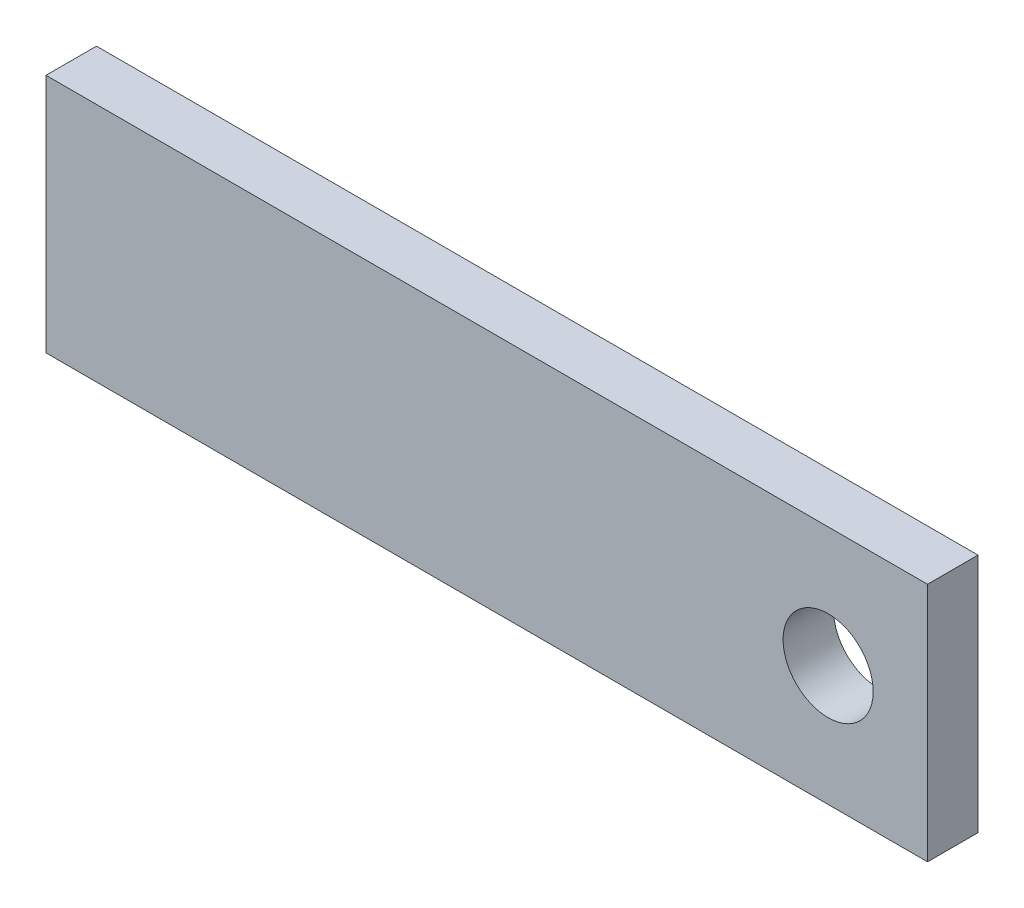
SolidWorks part; units mm, degrees
material "普通碳钢"
ref_plane "Front Plane" through (0, 0, 0) normal (0, 0, 1) x (1, 0, 0)
ref_plane "Top Plane" through (0, 0, 0) normal (0, 1, 0) x (1, 0, 0)
ref_plane "Right Plane" through (0, 0, 0) normal (1, 0, 0) x (0, 0, -1)
sketch "Sketch1" plane through (0, 0, 0) normal (0, 0, 1) x (1, 0, 0)
  line L1 (-123.952, 19.05) -> (15.748, 19.05)
  line L2 (-123.952, 19.05) -> (-123.952, -19.05)
  line L3 (-123.952, -19.05) -> (15.748, -19.05)
  line L4 (15.748, 19.05) -> (15.748, -19.05)
  circle A0 centre (0, 0) radius 7.1374
  dimension "D4" = 14.2748
  dimension "D1" = 139.7
  dimension "D2" = 38.1
  dimension "D3" = 19.05
  dimension "D5" = 15.748
extrude "Boss-Extrude1" add sketch "Sketch1" along normal mid plane 8
